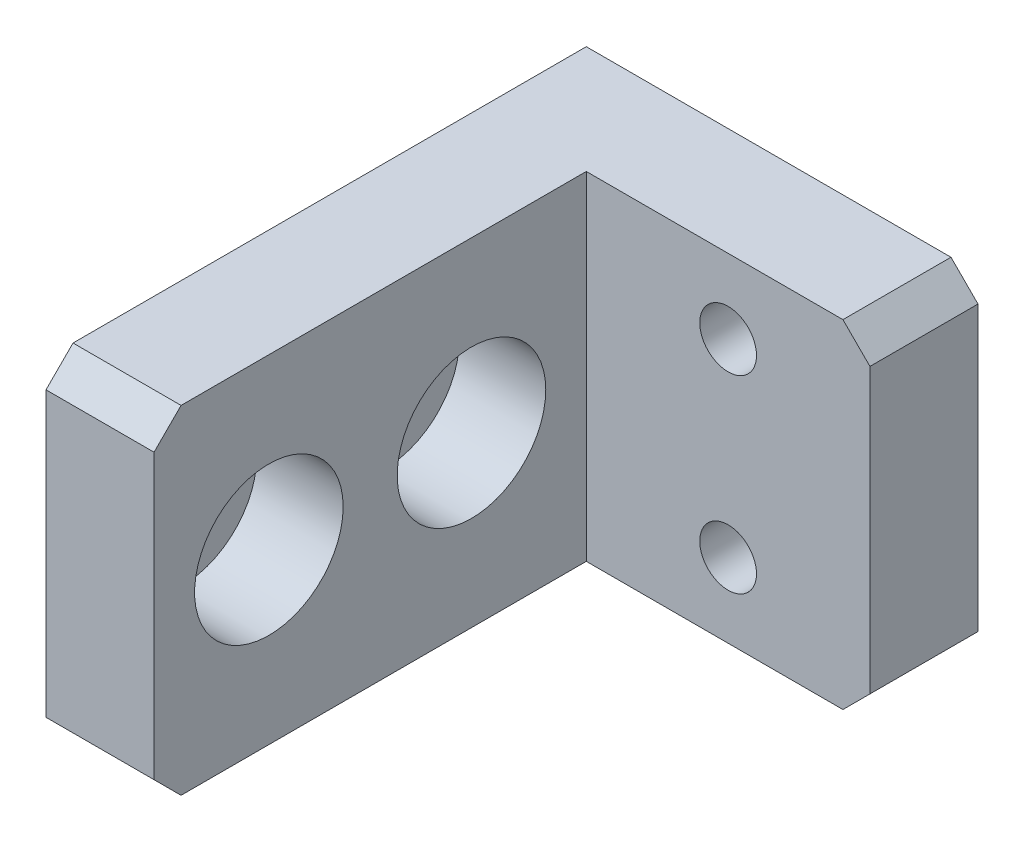
from build123d import *

# Parameters (mm, degrees)
EXTRUDE_1_DEPTH              = 12.5
HOLE_WIZARD_M5_1_D           = 4.2
HOLE_WIZARD_M6_1_D           = 6.6
HOLE_WIZARD_M6_1_CBORE_D     = 11
HOLE_WIZARD_M6_1_CBORE_DEPTH = 6.4
CHAMFER_1_SIZE               = 2


with BuildPart() as part:
    # 草图1 → 凸台-拉伸1 (new, symmetric)
    with BuildSketch(Plane(origin=(0, 0, 0), x_dir=(1, 0, 0), z_dir=(0, 1, 0))):
        Polygon((0, 0), (0, 32), (21, 32), (21, 40), (-8, 40), (-8, 0), align=None)
    extrude(amount=EXTRUDE_1_DEPTH, both=True)

    # M5 螺纹孔1 (through all)
    with Locations(Plane.XY.offset(-32)):
        with Locations((10.5, 7), (10.5, -7)):
            Hole(HOLE_WIZARD_M5_1_D / 2)

    # M6 六角凹头螺钉的柱形沉头孔1 (through all)
    with Locations(Plane(origin=(0, 0, 0), x_dir=(0, 0, -1), z_dir=(1, 0, 0))):
        with Locations((8.5, 0), (23.5, 0)):
            CounterBoreHole(HOLE_WIZARD_M6_1_D / 2, HOLE_WIZARD_M6_1_CBORE_D / 2, HOLE_WIZARD_M6_1_CBORE_DEPTH)

    # 倒角1
    chamfer_1_edges = [part.edges().sort_by_distance(p)[0] for p in [
        (21, 12.5, -36),
        (-4, 12.5, 0),
        (21, -12.5, -36),
        (-4, -12.5, 0),
    ]]
    chamfer(chamfer_1_edges, length=CHAMFER_1_SIZE)


solid = part.part
